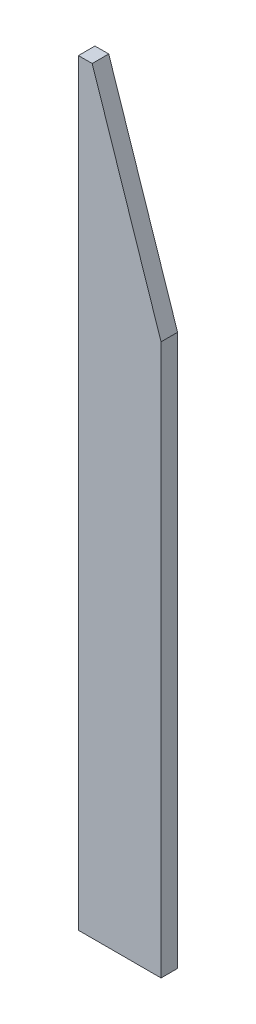
from build123d import *

# Parameters (mm, degrees)
SKETCH_1_W          = 60
SKETCH_1_H          = 550
EXTRUDE_1_DEPTH     = 12
CUT_EXTRUDE_1_DEPTH = 12


with BuildPart() as part:
    # 草图1 → 凸台-拉伸1 (new body)
    with BuildSketch(Plane.XY):
        Rectangle(SKETCH_1_W, SKETCH_1_H)
    extrude(amount=EXTRUDE_1_DEPTH)

    # 草图2 → 切除-拉伸1 (cut)
    with BuildSketch(Plane.XY.offset(12)):
        Polygon((-20, 275), (30, 125), (30, 275), align=None)
    extrude(amount=-CUT_EXTRUDE_1_DEPTH, mode=Mode.SUBTRACT)


solid = part.part
